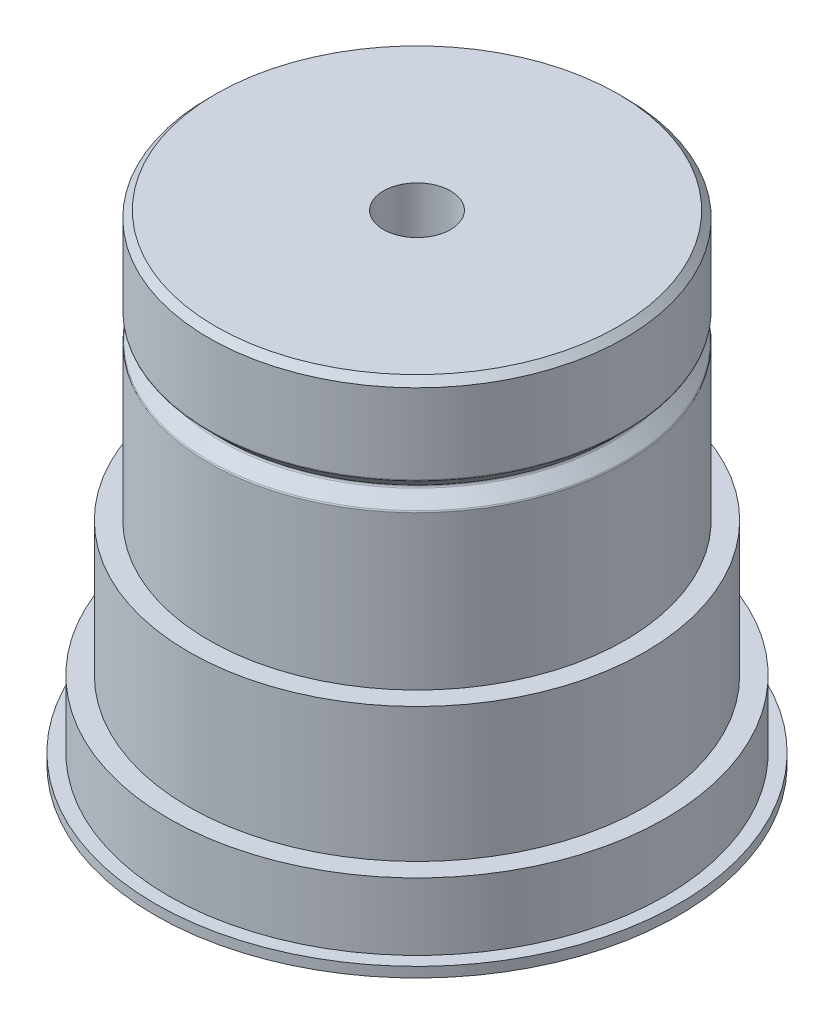
SolidWorks part; units mm, degrees
ref_plane "前视基准面" through (0, 0, 0) normal (0, 0, 1) x (1, 0, 0)
ref_plane "上视基准面" through (0, 0, 0) normal (0, 1, 0) x (1, 0, 0)
ref_plane "右视基准面" through (0, 0, 0) normal (1, 0, 0) x (0, 0, -1)
sketch "草图1" plane through (0, 0, 0) normal (0, 0, 1) x (1, 0, 0)
  line L0 (0, 0) -> (0, 83.358) construction
  line L1 (-12.5, 0) -> (-12.5, 25)
  line L2 (-12.5, 25) -> (-5, 25)
  line L3 (-5, 25) -> (-5, 71.5)
  line L4 (-5, 71.5) -> (-31, 71.5)
  line L5 (-31, 71.5) -> (-31, 31.5) construction
  line L6 (-31, 31.5) -> (-34, 31.5)
  line L7 (-34, 31.5) -> (-34, 11.5)
  line L8 (-34, 11.5) -> (-37, 11.5)
  line L9 (-37, 11.5) -> (-37, 1.5)
  line L10 (-37, 1.5) -> (-39, 1.5)
  line L11 (-39, 1.5) -> (-39, 0)
  line L12 (-39, 0) -> (-12.5, 0)
  line L13 (-31, 71.5) -> (-31, 58.6243)
  line L14 (-30.9121, 58.4121) -> (-29.2121, 56.7121)
  line L15 (-29.2121, 56.2879) -> (-30.9121, 54.5879)
  line L16 (-31, 54.3757) -> (-31, 31.5)
  arc A0 (-31, 58.6243) -> (-30.9121, 58.4121) centre (-30.7, 58.6243) ccw
  arc A1 (-30.9121, 54.5879) -> (-31, 54.3757) centre (-30.7, 54.3757) ccw
  arc A2 (-29.2121, 56.7121) -> (-29.2121, 56.2879) centre (-29.4243, 56.5) cw
  point P20 (-31, 58.5)
  point P23 (-31, 54.5)
  point P26 (-29, 56.5)
  dimension "D14" = 0.3
  dimension "D1" = 78
  dimension "D2" = 1.5
  dimension "D3" = 25
  dimension "D4" = 10
  dimension "D5" = 2
  dimension "D6" = 25
  dimension "D7" = 10
  dimension "D8" = 3
  dimension "D9" = 3
  dimension "D10" = 20
  dimension "D11" = 2
  dimension "D12" = 15
  dimension "D13" = 40
revolve "旋转1" add sketch "草图1" angle 360 about L0
chamfer "倒角1" distance 1 angle 45 1 edges at (0, 71.5, -31)
equation "\"图号代码1\"= \"图号代码\""
equation "\"名称代码2\"= \"名称代码\""
